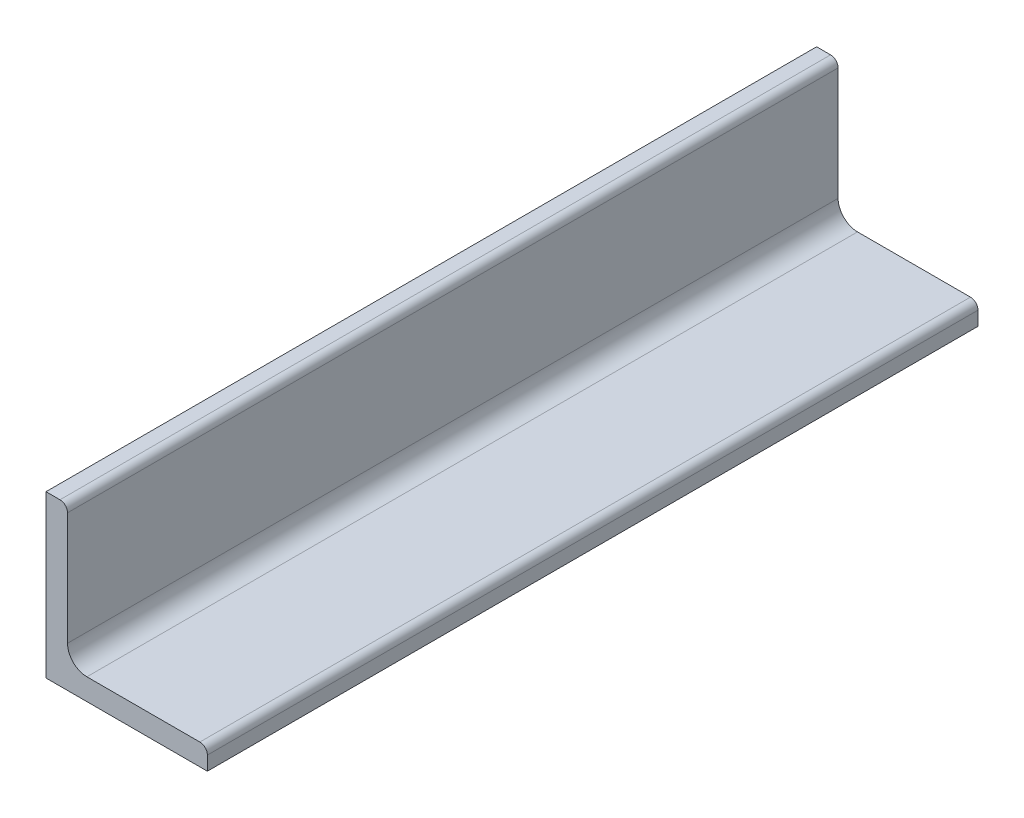
SolidWorks part; units mm, degrees
material "普通碳钢"
ref_plane "Front Plane" through (0, 0, 0) normal (0, 0, 1) x (1, 0, 0)
ref_plane "Top Plane" through (0, 0, 0) normal (0, 1, 0) x (1, 0, 0)
ref_plane "Right Plane" through (0, 0, 0) normal (1, 0, 0) x (0, 0, -1)
sketch "Sketch1" plane through (0, 0, 0) normal (0, 0, 1) x (1, 0, 0)
  line L0 (0, 75) -> (0, 0)
  line L1 (0, 0) -> (75, 0)
  line L2 (75, 0) -> (75, 6.5)
  line L3 (71.5, 10) -> (19, 10)
  line L4 (10, 19) -> (10, 71.5)
  line L5 (6.5, 75) -> (0, 75)
  arc A0 (19, 10) -> (10, 19) centre (19, 19) cw
  arc A1 (75, 6.5) -> (71.5, 10) centre (71.5, 6.5) ccw
  arc A2 (10, 71.5) -> (6.5, 75) centre (6.5, 71.5) ccw
  point P11 (75, 10)
  point P14 (10, 75)
  dimension "D5" = 9
  dimension "D6" = 3.5
  dimension "D1" = 75
  dimension "D2" = 75
  dimension "D3" = 10
  dimension "D4" = 10
extrude "Boss-Extrude1" add sketch "Sketch1" along normal mid plane 358.1
